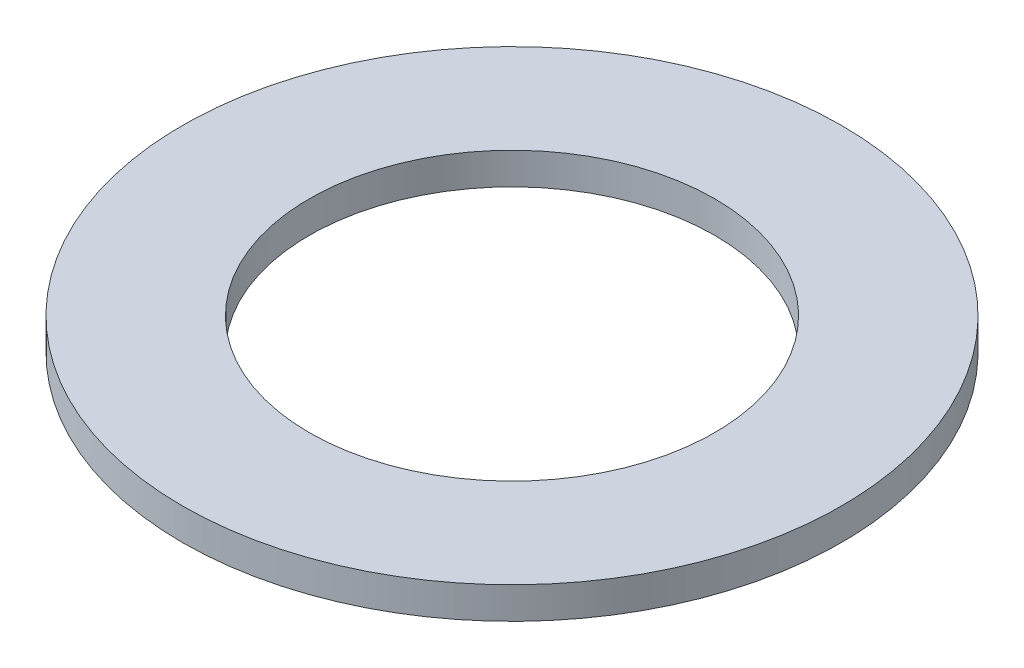
SolidWorks part; units mm, degrees
ref_plane "前视基准面" through (0, 0, 0) normal (0, 0, 1) x (1, 0, 0)
ref_plane "上视基准面" through (0, 0, 0) normal (0, 1, 0) x (1, 0, 0)
ref_plane "右视基准面" through (0, 0, 0) normal (1, 0, 0) x (0, 0, -1)
sketch "草图1" plane through (0, 0, 0) normal (0, 1, 0) x (1, 0, 0)
  circle A0 centre (0, 0) radius 155.82
  circle A1 centre (0, 0) radius 95.82
  dimension "D1" = 311.64
  dimension "D2" = 191.64
extrude "凸台-拉伸1" add sketch "草图1" along normal blind 15 contours A0 | A1
